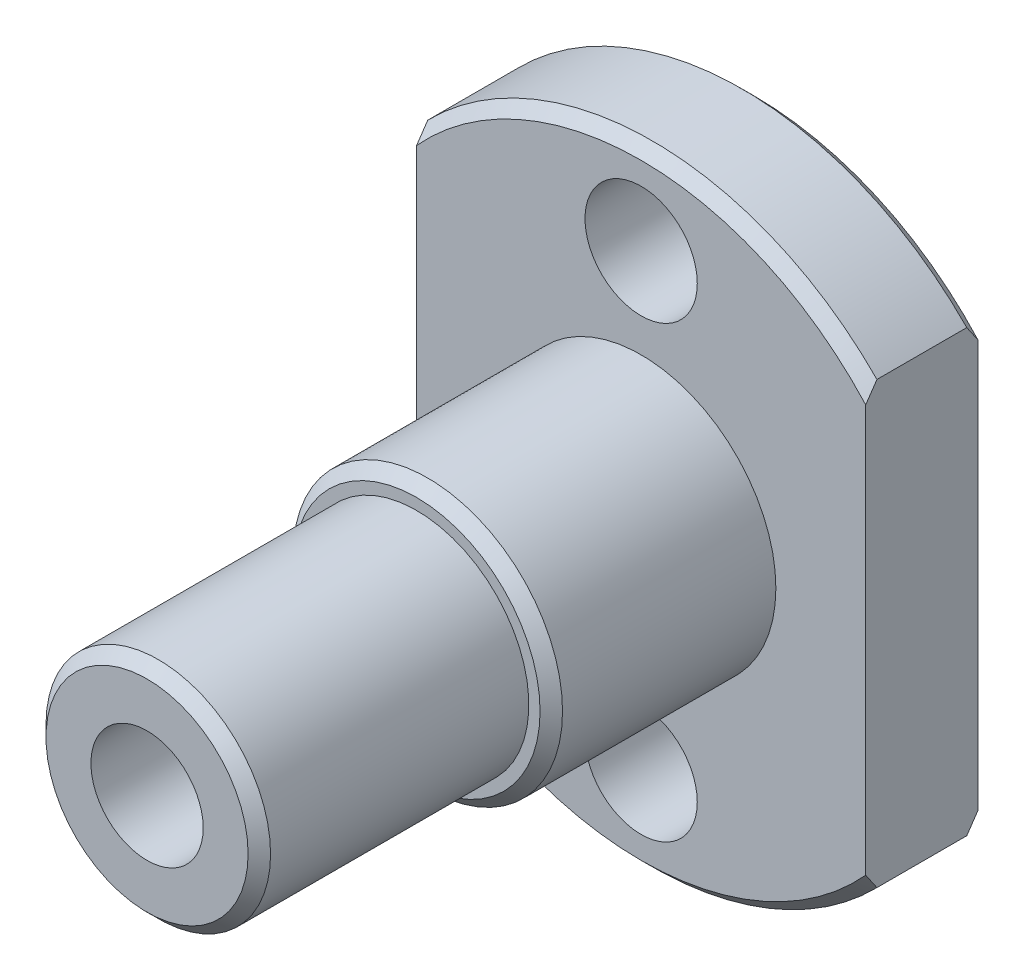
SolidWorks part; units mm, degrees
ref_plane "前视基准面" through (0, 0, 0) normal (0, 0, 1) x (1, 0, 0)
ref_plane "上视基准面" through (0, 0, 0) normal (0, 1, 0) x (1, 0, 0)
ref_plane "右视基准面" through (0, 0, 0) normal (1, 0, 0) x (0, 0, -1)
sketch "草图1" plane through (0, 0, 0) normal (0, 0, 1) x (1, 0, 0)
  circle A0 centre (0, 0) radius 5
  dimension "D1" = 10
extrude "凸台-拉伸1" add sketch "草图1" along normal blind 22
sketch "草图2" plane through (0, 0, 0) normal (0, 0, -1) x (-1, 0, 0)
  circle A0 centre (0, 0) radius 6
  dimension "D1" = 12
extrude "凸台-拉伸2" add sketch "草图2" against normal blind 10
sketch "草图3" plane through (0, 0, 0) normal (0, 0, -1) x (-1, 0, 0)
  circle A0 centre (0, 0) radius 14
  dimension "D1" = 28
extrude "凸台-拉伸3" add sketch "草图3" along normal blind 5
sketch "草图4" plane through (0, 0, -5) normal (0, 0, -1) x (-1, 0, 0)
  line L0 (0, 0) -> (0, 25.9804) construction
  line L1 (-10, 18.6438) -> (10, 18.6438)
  line L2 (-10, 18.6438) -> (-10, -19.0977)
  line L3 (-10, -19.0977) -> (10, -19.0977)
  line L4 (10, 18.6438) -> (10, -19.0977)
  dimension "D1" = 20
extrude "切除-拉伸1" cut sketch "草图4" against normal blind 5 flip side to cut
hole_wizard "Ø5.0 (5) 直径孔1" positions "草图6" profile "草图5" hole size "Ø5.0" standard "GB"
sketch "草图6" plane through (0, 0, 0) normal (0, 0, 1) x (1, 0, 0)
  line L0 (10, 0) -> (-16.1274, 0) construction
  line L1 (10, 9.798) -> (10, -9.798) construction
  line L3 (0, 0) -> (0, -27.4516) construction
  point P0 (0, 10)
  point P2 (0, -10)
  dimension "D1" = 20
sketch "草图5" plane through (0, 10, 0) normal (1, 0, 0) x (0, -1, 0)
  line L0 (0, 0) -> (0, 21.5022)
  line L1 (0, 21.5022) -> (2.5, 20)
  line L2 (2.5, 20) -> (2.5, 0)
  line L5 (2.5, 0) -> (0, 0)
  line L10 (0, 21.5022) -> (-2.5, 20) construction
  line L11 (0, -6.35) -> (0, 107.95) construction
  dimension "孔直径" = 5
  dimension "孔深度" = 20
  dimension "导头角度" = 118
hole_wizard "M6 螺纹孔1" positions "草图8" profile "草图9" tap size "M6" standard "GB"
sketch "草图8" plane through (0, 0, 22) normal (0, 0, 1) x (1, 0, 0)
  point P0 (0, 0)
sketch "草图9" plane through (0, 0, 22) normal (1, 0, 0) x (0, -1, 0)
  line L0 (0, 0) -> (0, 16.5022)
  line L1 (0, 16.5022) -> (2.5, 15)
  line L2 (2.5, 15) -> (2.5, 0)
  line L5 (2.5, 0) -> (0, 0)
  line L10 (0, 16.5022) -> (-2.5, 15) construction
  line L11 (0, -6.35) -> (0, 107.95) construction
  dimension "螺纹孔钻头直径" = 5
  dimension "螺纹孔钻头深度" = 15
  dimension "导头角度" = 118
cosmetic thread "孔螺蚊线1"
chamfer "倒角1" distance 0.5 angle 45 2 edges at (-6, 0, 10) (5, 0, 22)
chamfer "倒角2" distance 0.5 angle 45 4 edges at (0, 14, -5) (0, -14, -5) (0, 14, 0) (0, -14, 0)
